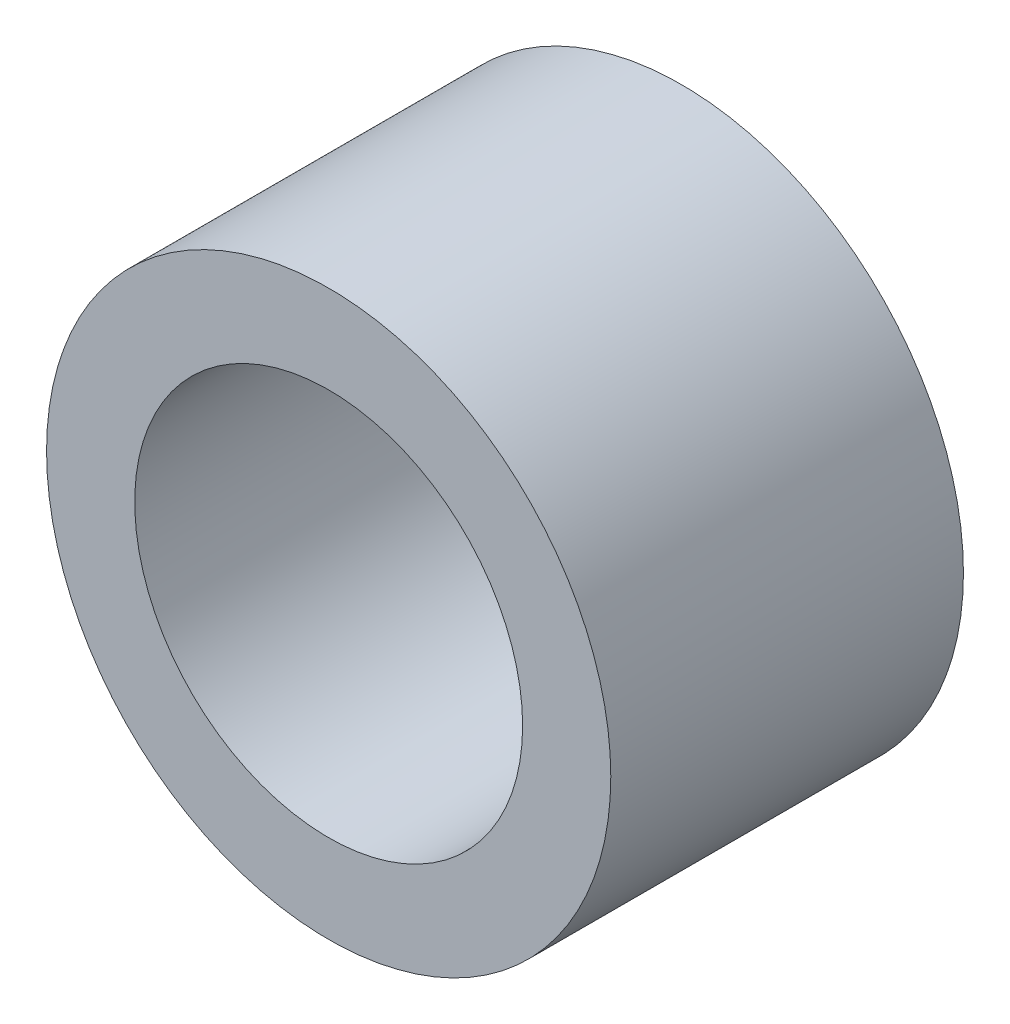
from build123d import *

# Parameters (mm, degrees)
SKETCH_1_R      = 12
SKETCH_1_R_2    = 8.25
EXTRUDE_1_DEPTH = 15


with BuildPart() as part:
    # 草图1 → 凸台-拉伸1 (new body)
    with BuildSketch(Plane.XY):
        Circle(SKETCH_1_R)
        Circle(SKETCH_1_R_2, mode=Mode.SUBTRACT)
    extrude(amount=EXTRUDE_1_DEPTH)


solid = part.part
